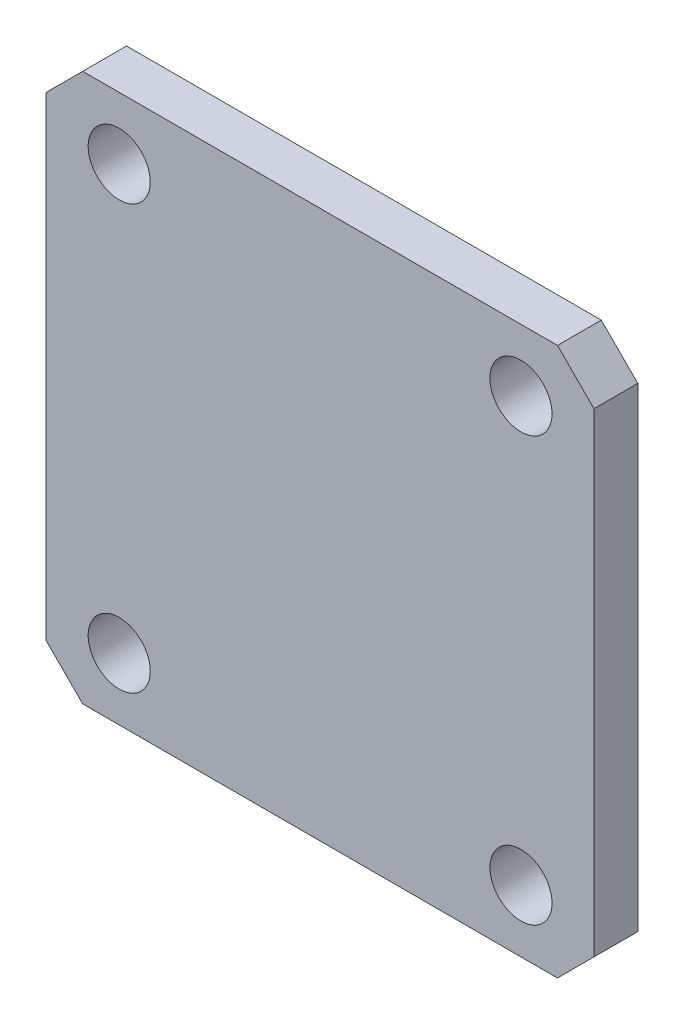
from build123d import *

# Parameters (mm, degrees)
SKETCH1_R           = 4.25
BOSS_EXTRUDE1_DEPTH = 6


with BuildPart() as part:
    # Sketch1 → Boss-Extrude1 (new body)
    with BuildSketch(Plane.XY):
        Polygon((-37.5, 32.5), (-32.5, 37.5), (32.5, 37.5), (37.5, 32.5), (37.5, -32.5), (32.5, -37.5), (-32.5, -37.5), (-37.5, -32.5), align=None)
        with Locations((-27.5, 29)):
            Circle(SKETCH1_R, mode=Mode.SUBTRACT)
        with Locations((27.5, 29)):
            Circle(SKETCH1_R, mode=Mode.SUBTRACT)
        with Locations((-27.5, -29)):
            Circle(SKETCH1_R, mode=Mode.SUBTRACT)
        with Locations((27.5, -29)):
            Circle(SKETCH1_R, mode=Mode.SUBTRACT)
    extrude(amount=BOSS_EXTRUDE1_DEPTH)


solid = part.part
